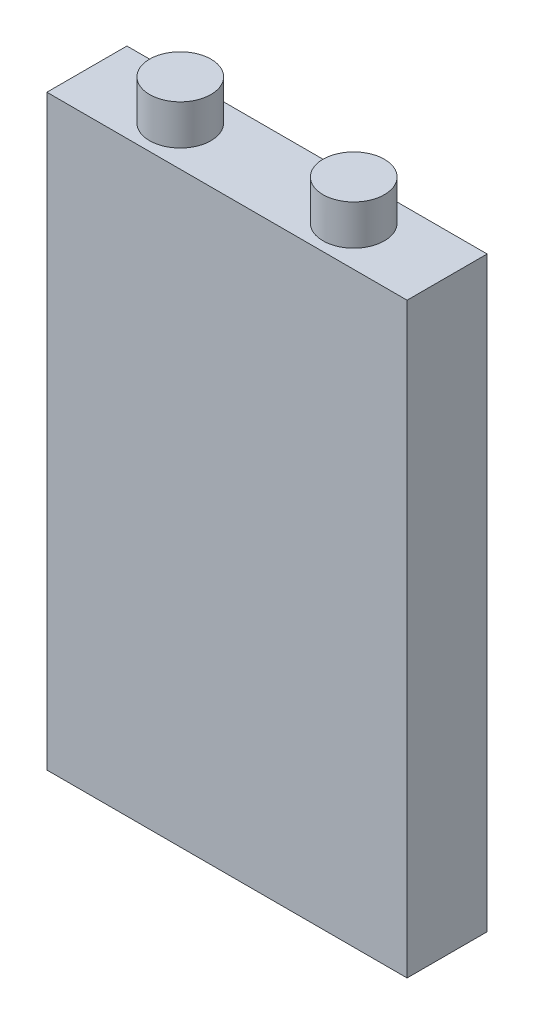
from build123d import *

# Parameters (mm, degrees)
SKETCH1_W           = 135
SKETCH1_H           = 220
BOSS_EXTRUDE1_DEPTH = 15
SKETCH2_R           = 11.5
BOSS_EXTRUDE2_DEPTH = 15


with BuildPart() as part:
    # Sketch1 → Boss-Extrude1 (new, symmetric)
    with BuildSketch(Plane.XY):
        Rectangle(SKETCH1_W, SKETCH1_H)
    extrude(amount=BOSS_EXTRUDE1_DEPTH, both=True)

    # Sketch2 → Boss-Extrude2 (add)
    with BuildSketch(Plane(origin=(0, 110, 0), x_dir=(1, 0, 0), z_dir=(0, 1, 0))):
        with Locations((32.5, 0)):
            Circle(SKETCH2_R)
        with Locations((-32.5, 0)):
            Circle(SKETCH2_R)
    extrude(amount=BOSS_EXTRUDE2_DEPTH)


solid = part.part
